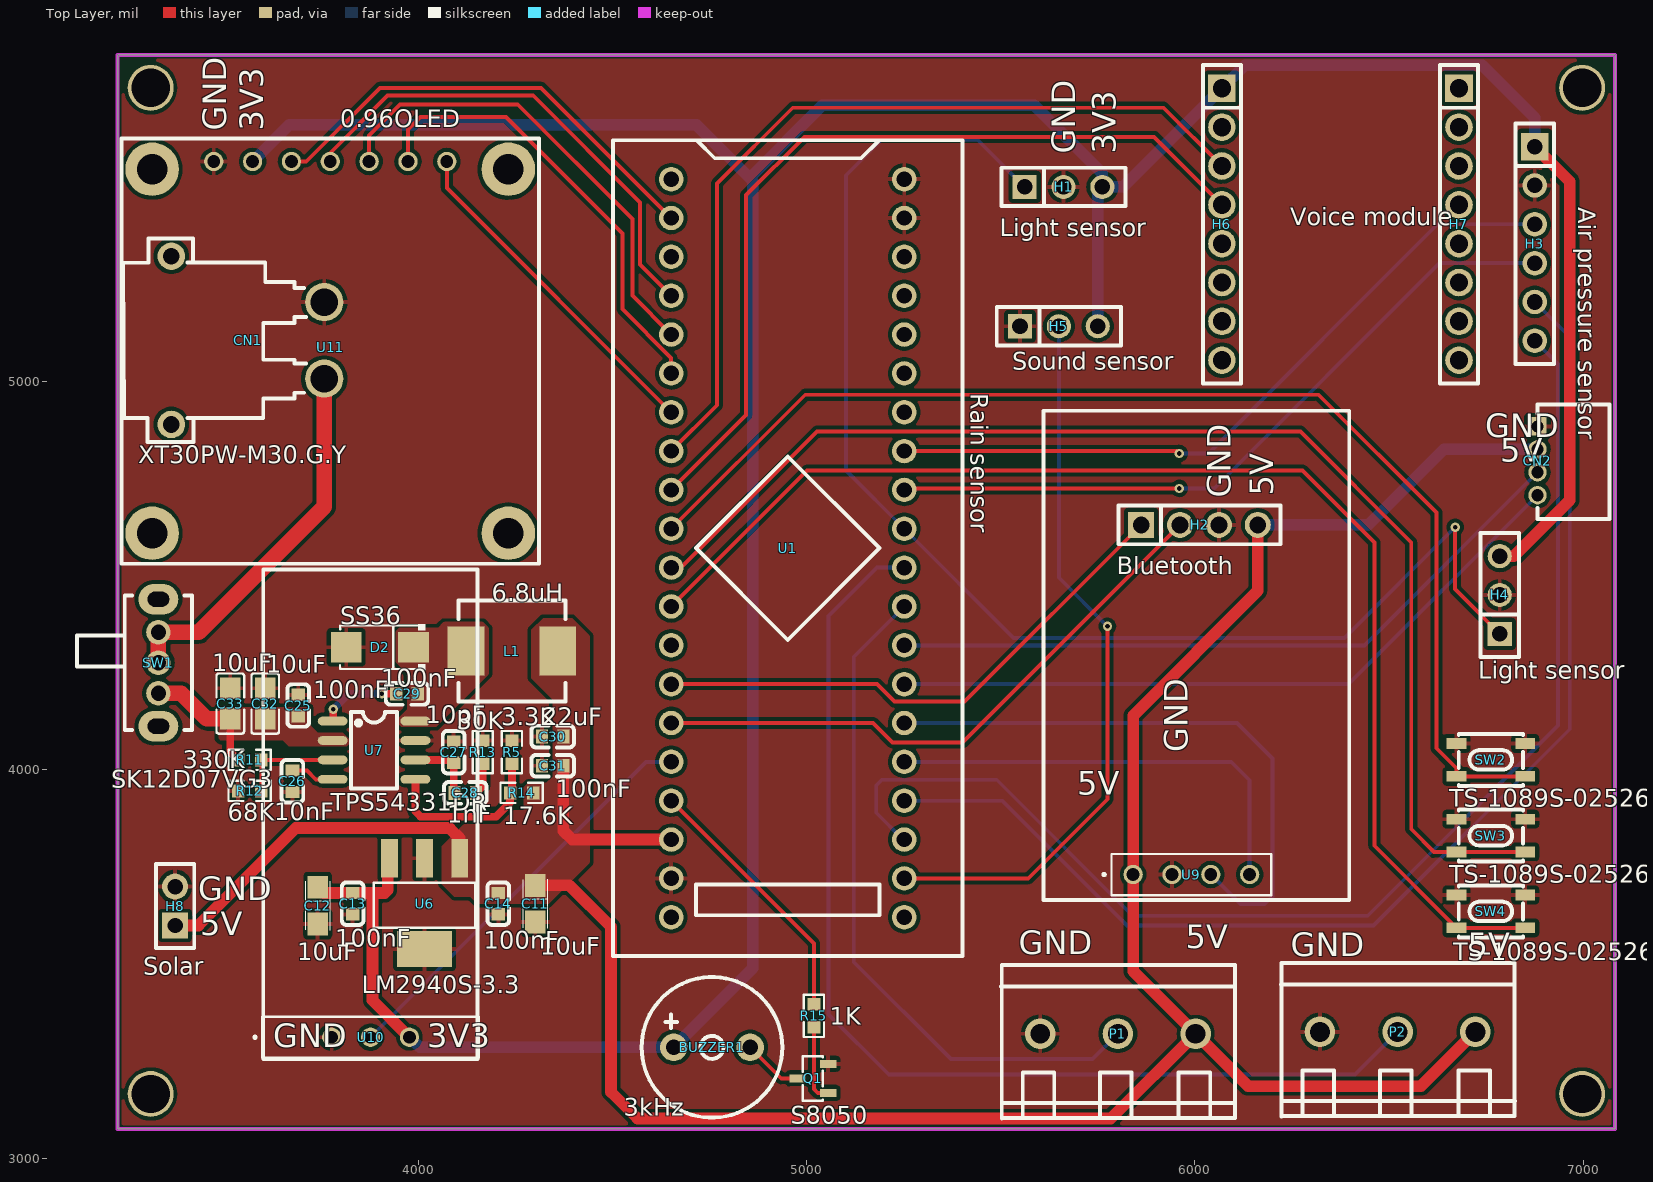
[diagram p0: Top Layer view]
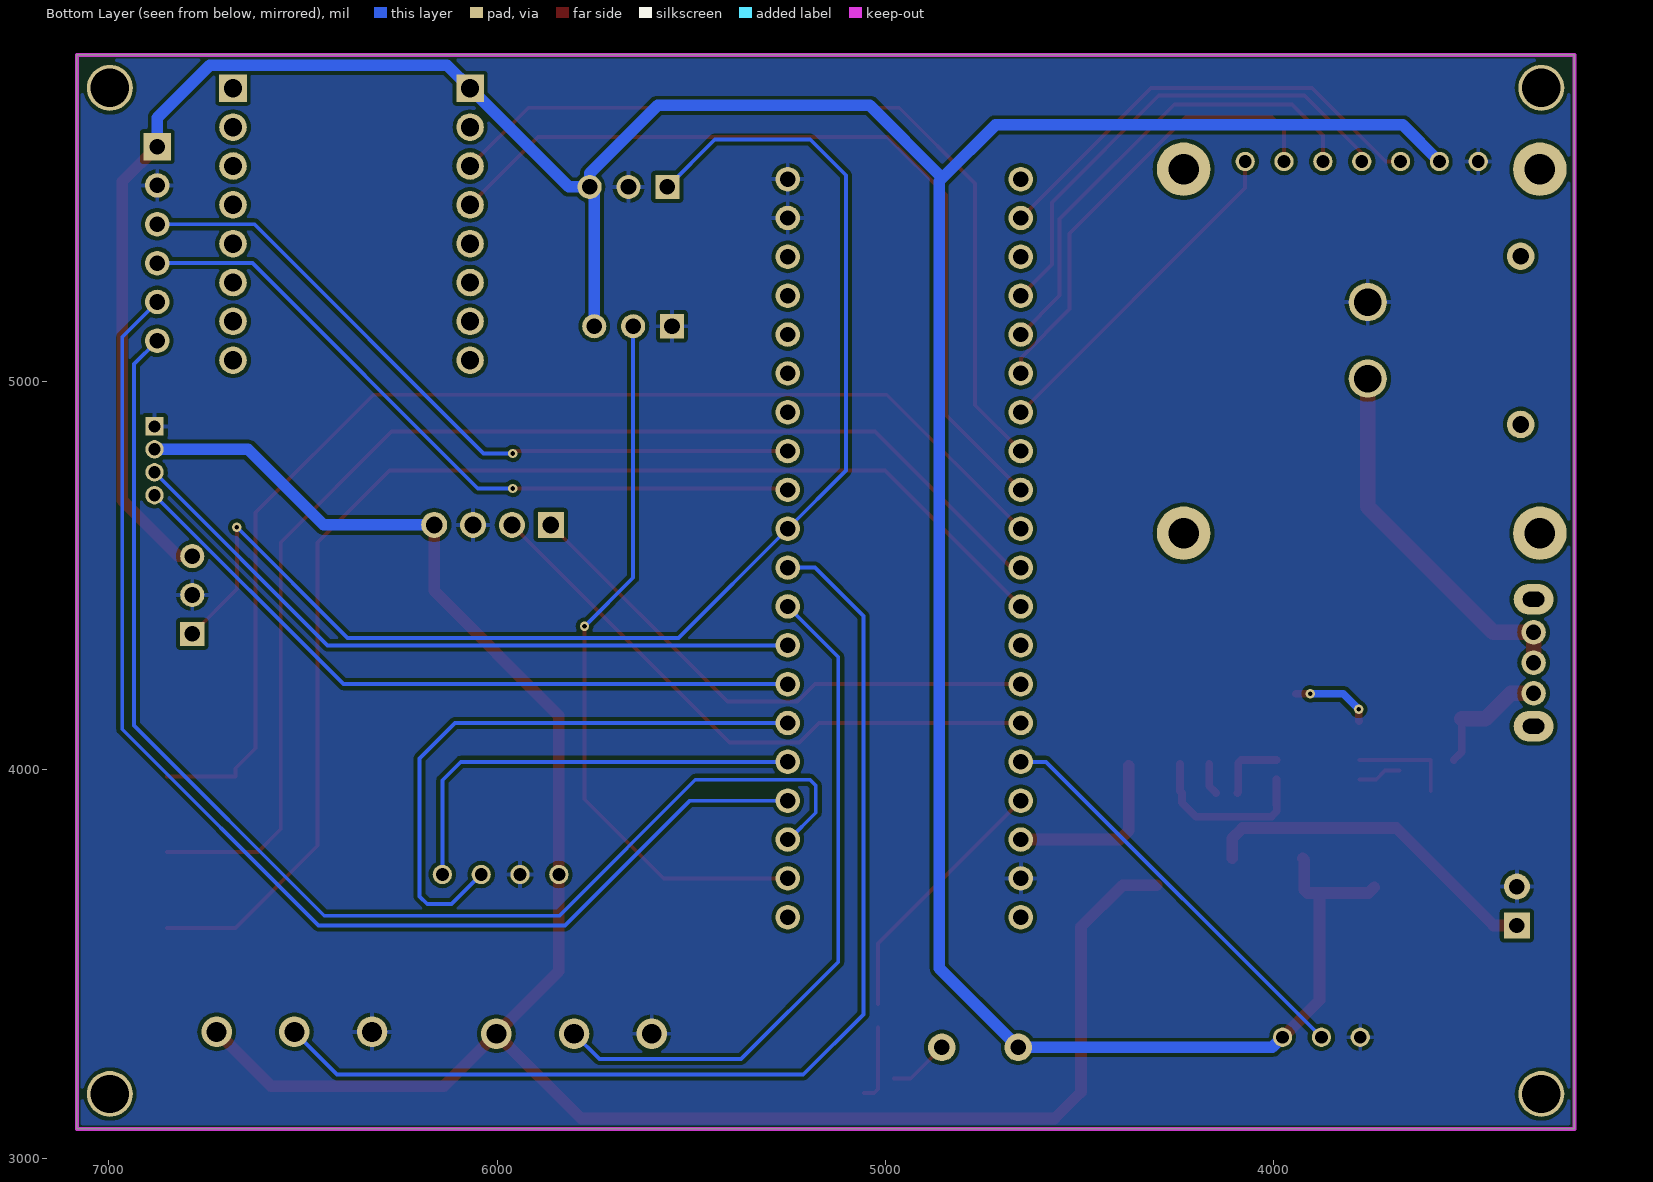
[diagram p1: Bottom Layer view, seen from below]
# Altium PCB MISC64781.pcbdoc
Units mil, origin at the board's own origin, x right, y up, seen from the top; angles counter-clockwise.
Board outline 3855 x 2765 mil, 2 copper layers (Top Layer, Bottom Layer), stack 62.206 mil thick; 45 components, 45 nets, 189 pads, 6 vias.

## Layer stack, top to bottom
Top Solder Mask Layer: solder mask 0.394, Dk 3.3
Top Layer: signal copper 1.379
Dielectric1: surface 59.449, FR4, Dk 4.5
Bottom Layer: signal copper 1.378
Bottom Solder Mask Layer: solder mask 0.394, Dk 3.3

## Board outline
3226.76,5840 3226.76,3075 7081.76,3075 7081.76,5840

## Design rules (kind name [scope] priority, off if disabled: settings)
BoardOutlineClearance copperThickness2oz_1 [All] p2 off: genericclearance=7.99 ignorepadtopadclearanceinfootprint=FALSE except(0: Arc-SplitContinuation Track-SplitContinuation SMDPad-SplitContinuation THPad-SplitContinuation Via-SplitContinuation Fill-SplitContinuation Region-SplitContinuation Poly-SplitContinuation Text-SplitContinuation Hole-SplitContinuation; 5.98: Arc-CutoutEdge Track-CutoutEdge SMDPad-CutoutEdge THPad-CutoutEdge Via-CutoutEdge Text-CutoutEdge; 6.89: Hole-OutlineEdge Hole-CutoutEdge; 10: Poly-OutlineEdge Poly-CutoutEdge; 11.81: Arc-OutlineEdge Track-OutlineEdge SMDPad-OutlineEdge THPad-OutlineEdge Via-OutlineEdge Fill-OutlineEdge Region-OutlineEdge Text-OutlineEdge Fill-CutoutEdge Region-CutoutEdge)
BoardOutlineClearance Plane_innerPlane_1 [All] p4 off: genericclearance=4.02 ignorepadtopadclearanceinfootprint=FALSE except(0: Arc-SplitContinuation Track-SplitContinuation SMDPad-SplitContinuation THPad-SplitContinuation Via-SplitContinuation Fill-SplitContinuation Region-SplitContinuation Poly-SplitContinuation Text-SplitContinuation Hole-SplitContinuation; 5.98: Arc-CutoutEdge Track-CutoutEdge SMDPad-CutoutEdge THPad-CutoutEdge Via-CutoutEdge Text-CutoutEdge; 6.89: Hole-OutlineEdge Hole-CutoutEdge; 10: Poly-OutlineEdge Poly-CutoutEdge; 11.81: Arc-OutlineEdge Track-OutlineEdge SMDPad-OutlineEdge THPad-OutlineEdge Via-OutlineEdge Fill-OutlineEdge Region-OutlineEdge Text-OutlineEdge Fill-CutoutEdge Region-CutoutEdge)
BoardOutlineClearance Copper_copperRegion_1 [All] p6 off: genericclearance=4.02 ignorepadtopadclearanceinfootprint=FALSE except(0: Arc-SplitContinuation Track-SplitContinuation SMDPad-SplitContinuation THPad-SplitContinuation Via-SplitContinuation Fill-SplitContinuation Region-SplitContinuation Poly-SplitContinuation Text-SplitContinuation Hole-SplitContinuation; 5.98: Arc-CutoutEdge Track-CutoutEdge SMDPad-CutoutEdge THPad-CutoutEdge Via-CutoutEdge Text-CutoutEdge; 6.89: Hole-OutlineEdge Hole-CutoutEdge; 10: Poly-OutlineEdge Poly-CutoutEdge; 11.81: Arc-OutlineEdge Track-OutlineEdge SMDPad-OutlineEdge THPad-OutlineEdge Via-OutlineEdge Fill-OutlineEdge Region-OutlineEdge Text-OutlineEdge Fill-CutoutEdge Region-CutoutEdge)
BoardOutlineClearance Copper_电源_1 [All] p8 off: genericclearance=4.02 ignorepadtopadclearanceinfootprint=FALSE except(0: Arc-SplitContinuation Track-SplitContinuation SMDPad-SplitContinuation THPad-SplitContinuation Via-SplitContinuation Fill-SplitContinuation Region-SplitContinuation Poly-SplitContinuation Text-SplitContinuation Hole-SplitContinuation; 5.98: Arc-CutoutEdge Track-CutoutEdge SMDPad-CutoutEdge THPad-CutoutEdge Via-CutoutEdge Text-CutoutEdge; 6.89: Hole-OutlineEdge Hole-CutoutEdge; 10: Poly-OutlineEdge Poly-CutoutEdge; 11.81: Arc-OutlineEdge Track-OutlineEdge SMDPad-OutlineEdge THPad-OutlineEdge Via-OutlineEdge Fill-OutlineEdge Region-OutlineEdge Text-OutlineEdge Fill-CutoutEdge Region-CutoutEdge)
BoardOutlineClearance copperThickness1oz_1 [All] p10: genericclearance=4.02 ignorepadtopadclearanceinfootprint=FALSE except(0: Arc-SplitContinuation Track-SplitContinuation SMDPad-SplitContinuation THPad-SplitContinuation Via-SplitContinuation Fill-SplitContinuation Region-SplitContinuation Poly-SplitContinuation Text-SplitContinuation Hole-SplitContinuation; 5.98: Arc-CutoutEdge Track-CutoutEdge SMDPad-CutoutEdge THPad-CutoutEdge Via-CutoutEdge Text-CutoutEdge; 6.89: Hole-OutlineEdge Hole-CutoutEdge; 10: Poly-OutlineEdge Poly-CutoutEdge; 11.81: Arc-OutlineEdge Track-OutlineEdge SMDPad-OutlineEdge THPad-OutlineEdge Via-OutlineEdge Fill-OutlineEdge Region-OutlineEdge Text-OutlineEdge Fill-CutoutEdge Region-CutoutEdge)
Clearance copperThickness2oz [All] p1 off: gap=7.99 ignorepadtopadclearanceinfootprint=FALSE except(5.98: SMDPad-Track SMDPad-SMDPad THPad-Track SMDPad-THPad THPad-THPad Track-Via SMDPad-Via THPad-Via Via-Via Fill-SMDPad Region-SMDPad Fill-THPad Region-THPad Fill-Via Region-Via Fill-Fill Fill-Region Region-Region Arc-Track Arc-SMDPad Arc-THPad Arc-Via Fill-Arc Region-Arc Arc-Arc Text-Track SMDPad-Text Text-THPad Text-Via Fill-Text Region-Text Arc-Text Text-Text; 6.89: Hole-Track Hole-SMDPad Hole-THPad Hole-Via Fill-Hole Region-Hole Hole-Arc Hole-Text; 10: Poly-Track Poly-SMDPad Poly-THPad Poly-Via Poly-Fill Poly-Region Poly-Poly Poly-Arc Poly-Text Poly-Hole; 11.81: Fill-Track Region-Track)
Clearance Plane_innerPlane [All] p3 off: gap=4.02 ignorepadtopadclearanceinfootprint=FALSE except(5.98: SMDPad-Track SMDPad-SMDPad THPad-Track SMDPad-THPad THPad-THPad Track-Via SMDPad-Via THPad-Via Via-Via Fill-SMDPad Region-SMDPad Fill-THPad Region-THPad Fill-Via Region-Via Fill-Fill Fill-Region Region-Region Arc-Track Arc-SMDPad Arc-THPad Arc-Via Fill-Arc Region-Arc Arc-Arc Text-Track SMDPad-Text Text-THPad Text-Via Fill-Text Region-Text Arc-Text Text-Text; 6.89: Hole-Track Hole-SMDPad Hole-THPad Hole-Via Fill-Hole Region-Hole Hole-Arc Hole-Text; 10: Poly-Track Poly-SMDPad Poly-THPad Poly-Via Poly-Fill Poly-Region Poly-Poly Poly-Arc Poly-Text Poly-Hole; 11.81: Fill-Track Region-Track)
Clearance Copper_copperRegion [All] p5 off: gap=4.02 ignorepadtopadclearanceinfootprint=FALSE except(5.98: SMDPad-Track SMDPad-SMDPad THPad-Track SMDPad-THPad THPad-THPad Track-Via SMDPad-Via THPad-Via Via-Via Fill-SMDPad Region-SMDPad Fill-THPad Region-THPad Fill-Via Region-Via Fill-Fill Fill-Region Region-Region Arc-Track Arc-SMDPad Arc-THPad Arc-Via Fill-Arc Region-Arc Arc-Arc Text-Track SMDPad-Text Text-THPad Text-Via Fill-Text Region-Text Arc-Text Text-Text; 6.89: Hole-Track Hole-SMDPad Hole-THPad Hole-Via Fill-Hole Region-Hole Hole-Arc Hole-Text; 10: Poly-Track Poly-SMDPad Poly-THPad Poly-Via Poly-Fill Poly-Region Poly-Poly Poly-Arc Poly-Text Poly-Hole; 11.81: Fill-Track Region-Track)
Clearance Copper_电源 [All] p7 off: gap=4.02 ignorepadtopadclearanceinfootprint=FALSE except(5.98: SMDPad-Track SMDPad-SMDPad THPad-Track SMDPad-THPad THPad-THPad Track-Via SMDPad-Via THPad-Via Via-Via Fill-SMDPad Region-SMDPad Fill-THPad Region-THPad Fill-Via Region-Via Fill-Fill Fill-Region Region-Region Arc-Track Arc-SMDPad Arc-THPad Arc-Via Fill-Arc Region-Arc Arc-Arc Text-Track SMDPad-Text Text-THPad Text-Via Fill-Text Region-Text Arc-Text Text-Text; 6.89: Hole-Track Hole-SMDPad Hole-THPad Hole-Via Fill-Hole Region-Hole Hole-Arc Hole-Text; 10: Poly-Track Poly-SMDPad Poly-THPad Poly-Via Poly-Fill Poly-Region Poly-Poly Poly-Arc Poly-Text Poly-Hole; 11.81: Fill-Track Region-Track)
Clearance copperThickness1oz [All] p9: gap=4.02 ignorepadtopadclearanceinfootprint=FALSE except(5.98: SMDPad-Track SMDPad-SMDPad THPad-Track SMDPad-THPad THPad-THPad Track-Via SMDPad-Via THPad-Via Via-Via Fill-SMDPad Region-SMDPad Fill-THPad Region-THPad Fill-Via Region-Via Fill-Fill Fill-Region Region-Region Arc-Track Arc-SMDPad Arc-THPad Arc-Via Fill-Arc Region-Arc Arc-Arc Text-Track SMDPad-Text Text-THPad Text-Via Fill-Text Region-Text Arc-Text Text-Text; 6.89: Hole-Track Hole-SMDPad Hole-THPad Hole-Via Fill-Hole Region-Hole Hole-Arc Hole-Text; 10: Poly-Track Poly-SMDPad Poly-THPad Poly-Via Poly-Fill Poly-Region Poly-Poly Poly-Arc Poly-Text Poly-Hole; 11.81: Fill-Track Region-Track)
DiffPairsRouting differentialPair [All] p1: maxlimit=6 minlimit=6 mostfreqgap=6 toplayer_minwidth=5 toplayer_prefwidth=10 toplayer_maxwidth=100 toplayer_mingap=6 toplayer_prefgap=6 toplayer_maxgap=6 bottomlayer_minwidth=5 bottomlayer_prefwidth=10 bottomlayer_maxwidth=100 bottomlayer_mingap=6 bottomlayer_prefgap=6 bottomlayer_maxgap=6 maxuncoupledlength=10
HoleToHoleClearance otherClearance [All] p1: gap=11.81 allowstackedmicrovias=TRUE
Length netLength [All] p1: minlimit=0 maxlimit=0
PasteMaskExpansion pasteMaskExpansion [All] p1: expansion=0
PlaneConnect innerPlane [All] p1: planeconnectstyle=Relief reliefexpansion=20 reliefentries=4 reliefconductorwidth=10 reliefairgap=10
PolygonConnect 电源 [All] p1 off: connectstyle=Direct reliefconductorwidth=10 reliefentries=4 polygonreliefangle="90 Angle" airgapwidth=10 via.connectstyle=Relief via.reliefconductorwidth=10 via.reliefentries=4 via.polygonreliefangle="90 Angle" via.airgapwidth=10
PolygonConnect copperRegion [All] p2: connectstyle=Relief reliefconductorwidth=10 reliefentries=4 polygonreliefangle="90 Angle" airgapwidth=10 via.connectstyle=Relief via.reliefconductorwidth=10 via.reliefentries=4 via.polygonreliefangle="90 Angle" via.airgapwidth=10
RoutingVias viaSize [All] p1: holewidth=12.01 width=24.02 viastyle="Through Hole" minholewidth=11.81 minwidth=19.68 maxholewidth=248.03 maxwidth=393.7
SolderMaskExpansion solderMaskExpansion [IsVia] p1: expansion=-1000 istentingtop=TRUE
SolderMaskExpansion solderMaskExpansion [All] p2: expansion=2.01 istentingtop=FALSE
Width copperThickness2oz_2 [All] p1 off: maxlimit=100 minlimit=8 preferedwidth=10
Width copperThickness1oz_2 [All] p2: maxlimit=100 minlimit=5 preferedwidth=10

## Components (designator, comment, footprint, x,y, rotation, side; value= is the part's Value field where it differs from the comment)
BUZZER1 "3kHz" BUZ-TH_BD9.0-P5.00-D0.6-FD 4756.76,3285 r0 top
C11 "10uF" CASE-A_3216 4301.76,3655 r270 top
C12 "10uF" CASE-A_3216 3741.76,3650 r270 top
C13 "100nF" C0603 3831.76,3655 r90 top
C14 "100nF" C0603 4206.76,3655 r270 top
C25 "100nF" C0603 3691.76,4165 r270 top
C26 "10nF" C0603 3676.76,3970 r90 top
C27 "10pF" C0603 4091.76,4045 r270 top
C28 "1nF" C0603 4121.76,3940 r180 top
C29 "100nF" C0603 3971.76,4195 r0 top
C30 "22uF" C0603 4346.76,4085 r0 top
C31 "100nF" C0603 4346.76,4010 r0 top
C32 "10uF" C0805 3606.76,4170 r270 top
C33 "10uF" C0805 3516.76,4170 r270 top
CN1 "XT30PW-M30.G.Y" CONN-TH_XT30PW-M 3561.76,5105 r270 top
CN2 "PM2.5 sensor" CONN-TH_4P-P1.50_HCTL_HC-ZH1.5-4AW 6881.76,4795 r90 top
D2 "SS36" SMA_L4.3-W2.6-LS5.2-RD 3901.76,4315 r180 top
H1 "Light sensor" HDR-TH_3P-P2.54-V-F 5661.76,5500 r0 top
H2 "Bluetooth" HDR-TH_4P-P2.54-V-F 6011.76,4630 r0 top
H3 "Air pressure sensor" HDR-TH_6P-P2.54-V-F 6874.74,5353.84 r270 top
H4 "Light sensor" HDR-TH_3P-P2.54-V-F 6784.74,4449.51 r90 top
H5 "Sound sensor" HDR-TH_3P-P2.54-V-F 5649.74,5141.4 r0 top
H6 "Voice module" HDR-TH_8P-P2.54-V-F-1 6069.49,5403.84 r270 top
H7 "" HDR-TH_8P-P2.54-V-F-1 6679.74,5403.84 r270 top
H8 "Solar" HDR-TH_2P-P2.54-V-F 3374.74,3648.84 r90 top
L1 "6.8uH" IND-SMD_L7.0-W6.6 4241.76,4305 r0 top
P1 "Wind speed sensor" CONN-TH_3P-P5.00_WJ500V-5.08-3P 5801.76,3320 r0 top
P2 "Wind direction sensor" CONN-TH_3P-P5.00_WJ500V-5.08-3P 6521.76,3325 r0 top
Q1 "S8050" SOT-23-3_L2.9-W1.3-P1.90-LS2.3-BR 5016.76,3205 r0 top
R5 "3.3K" R0603 4241.76,4045 r270 top
R11 "330K" R0603 3566.76,4025 r180 top
R12 "68K" R0603 3566.76,3945 r0 top
R13 "30K" R0603 4166.76,4045 r270 top
R14 "17.6K" R0603 4266.76,3940 r0 top
R15 "1K" R0603 5019.16,3366.32 r270 top
SW1 "SK12D07VG3" SW-TH_SK12D07VG3 3331.76,4275 r270 top
SW2 "TS-1089S-02526" SW-SMD_4P-L4.2-W3.3-P2.15-LS5.1 6761.76,4025 r0 top
SW3 "TS-1089S-02526" SW-SMD_4P-L4.2-W3.3-P2.15-LS5.1 6761.76,3830 r0 top
SW4 "TS-1089S-02526" SW-SMD_4P-L4.2-W3.3-P2.15-LS5.1 6761.76,3635 r0 top
U1 "LCKFB-DKX-STM32F103C8T6" CONN-TH_L53.3-W22.9_STM32F103C8T6-CARD 4951.76,4570 r270 top
U6 "LM2940S-3.3" SOT-223-3_L6.5-W3.4-P2.30-LS7.0-BR 4016.76,3655 r90 top
U7 "TPS54331DR" SOIC-8_L5.0-W4.0-P1.27-LS6.0-BL 3886.76,4050 r270 top
U9 "Rain sensor" MQ-2烟雾传感器模块 5609.74,4923.84 r270 top
U10 "DHT11 temperature and humidity sensor" DHT11温湿度模块 3601.76,4515 r270 top
U11 "0.96OLED" 0.96寸OLED 3236.76,4530 r0 top

## Footprints (in the part's own frame and the unit in brackets; to place one, negate y for a bottom-side part, rotate by r counter-clockwise, add the part's x,y. Pads: shape width x height; smd on the part's side, far side on the other; paste and mask are expansions set on the pad)
0.96寸OLED [mm]
  round 1.26 hole 0.84: 1(6.03,26.3) 2(8.57,26.3) 3(11.11,26.3) 4(13.65,26.3) 5(16.19,26.3) 6(18.73,26.3) 7(21.27,26.3)
  round 3.5 hole 2: 8(2,25.8) 9(25.3,25.8) 10(2,2) 11(25.3,2)
  silkscreen extent 0,0 27.3,27.8
BUZ-TH_BD9.0-P5.00-D0.6-FD [mm]
  round 1.8 hole 1 copper offset 0,0: 1(-2.5,0)
  round 1.8 hole 1: 2(2.5,0)
  silkscreen extent -4.6,-4.6 4.6,4.6
C0603 [mm]
  rect 0.8x0.9 smd: 1(-0.7,0) 2(0.7,0)
  silkscreen extent -1.39,-0.71 1.39,0.71
C0805 [mm]
  rect 1.41x1.35 smd paste-100 mask+0.051: 1(-1,0) 2(1,0)
  silkscreen extent -1.96,-0.9 1.96,0.9
CASE-A_3216 [mil]
  rect 59.05x53.5 smd: 1(-47.24,0) 2(47.24,0)
  silkscreen extent -63,-32 63,32
CONN-TH_3P-P5.00_WJ500V-5.08-3P [mm]
  round 2 hole 1.3: 1(-5.08,0) 2(0,0) 3(5.08,0)
  silkscreen extent -7.64,-5.53 7.66,4.5
CONN-TH_4P-P1.50_HCTL_HC-ZH1.5-4AW [mm]
  round 1.2 hole 0.8 paste+0 mask+0.05: 1(-2.25,0) 2(-0.75,0) 3(0.75,0)
  rect 1.2x1.2 hole 0.8 paste+0 mask+0.05: 4(2.25,0)
  silkscreen extent -3.81,-4.7 3.68,0
CONN-TH_L53.3-W22.9_STM32F103C8T6-CARD [mm]
  round 1.6 hole 1: 1(-24.13,-7.62) 2(-21.59,-7.62) 3(-19.05,-7.62) 4(-16.51,-7.62) 5(-13.97,-7.62) 6(-11.43,-7.62) 7(-8.89,-7.62) 8(-6.35,-7.62) 9(-3.81,-7.62) 10(-1.27,-7.62) 11(1.27,-7.62) 12(3.81,-7.62) 13(6.35,-7.62) 14(8.89,-7.62) 15(11.43,-7.62) 16(13.97,-7.62) 17(16.51,-7.62) 18(19.05,-7.62) 19(21.59,-7.62) 20(24.13,-7.62) 21(24.13,7.62) 22(21.59,7.62) 23(19.05,7.62) 24(16.51,7.62) 25(13.97,7.62) 26(11.43,7.62) 27(8.89,7.62) 28(6.35,7.62) 29(3.81,7.62) 30(1.27,7.62) 31(-1.27,7.62) 32(-3.81,7.62) 33(-6.35,7.62) 34(-8.89,7.62) 35(-11.43,7.62) 36(-13.97,7.62) 37(-16.51,7.62) 38(-19.05,7.62) 39(-21.59,7.62) 40(-24.13,7.62)
  silkscreen extent -26.67,-11.43 26.67,11.43
CONN-TH_XT30PW-M [mm]
  round 2.5 hole 1.8: 1(-2.5,5) 2(2.5,5)
  round 1.8 hole 1.1: 3(5.5,-5) 4(-5.5,-5)
  silkscreen extent -6.65,-8.15 6.65,3.81
DHT11温湿度模块 [mil]
  round 49.61 hole 33.07: 1(1203.85,376.15) 2(1203.85,276.15) 3(1203.85,176.15)
  silkscreen extent 0,-28 1260,555
HDR-TH_2P-P2.54-V-F [mm]
  rect 1.7x1.7 hole 1: 1(-1.27,0)
  round 1.7 hole 1: 2(1.27,0)
  silkscreen extent -2.74,-1.25 2.74,1.25
HDR-TH_3P-P2.54-V-F [mil]
  rect 62x62 hole 40.16: 1(-100,0)
  round 62 hole 40.16: 2(0,0) 3(100,0)
  silkscreen extent -160,-49 160,49
HDR-TH_4P-P2.54-V-F [mm]
  rect 1.7x1.7 hole 1.1: 1(-3.81,0)
  round 1.7 hole 1.1: 2(-1.27,0) 3(1.27,0) 4(3.81,0)
  silkscreen extent -5.29,-1.27 5.29,1.27
HDR-TH_6P-P2.54-V-F [mm]
  rect 1.8x1.8 hole 1.02: 1(-6.35,0)
  round 1.6 hole 1.02: 2(-3.81,0) 3(-1.27,0) 4(1.27,0) 5(3.81,0) 6(6.35,0)
  silkscreen extent -7.87,-1.25 7.87,1.25
HDR-TH_8P-P2.54-V-F-1 [mm]
  rect 1.8x1.8 hole 1.2: 1(-8.89,0)
  round 1.8 hole 1.2: 2(-6.35,0) 3(-3.81,0) 4(-1.27,0) 5(1.27,0) 6(3.81,0) 7(6.35,0) 8(8.89,0)
  silkscreen extent -10.41,-1.25 10.41,1.25
IND-SMD_L7.0-W6.6 [mm]
  rect 2.4x3.2 smd: 1(-3,0) 2(3,0)
  silkscreen extent -3.5,-3.3 3.5,3.3
MQ-2烟雾传感器模块 [mil]
  round 49.61 hole 33.07: 1(1193.85,231.15) 2(1193.85,331.15) 3(1193.85,431.15) 4(1193.85,531.15)
  silkscreen extent 0,0 1260,787
R0603 [mil]
  rect 31.75x34.02 smd paste-3937.01 mask+2: 1(-29.66,0) 2(29.66,0)
  silkscreen extent -55,-26 55,26
SMA_L4.3-W2.6-LS5.2-RD [mm]
  rect 2x2 smd: 1(-2.2,0) 2(2.2,0)
  silkscreen extent -2.98,-1.5 2.6,1.5
SOIC-8_L5.0-W4.0-P1.27-LS6.0-BL [mil]
  oval 22.38x76.78 smd: 1(-75,-106.5) 2(-25,-106.5) 3(25,-106.5) 4(75,-106.5) 5(75,106.5) 6(25,106.5) 7(-25,106.5) 8(-75,106.5)
  silkscreen extent -98,-59 98,59
SOT-23-3_L2.9-W1.3-P1.90-LS2.3-BR [mm]
  rect 1.07x0.532 smd: 1(0.99,-0.95) 2(0.99,0.95) 3(-0.99,0)
  silkscreen extent -0.66,-1.45 0.64,1.45
SOT-223-3_L6.5-W3.4-P2.30-LS7.0-BR [mm]
  rect 2.5x1.1 smd: 1(2.97,-2.3) 2(2.97,0) 3(2.97,2.3)
  rect 2.34x3.6 smd: 4(-2.97,0)
  silkscreen extent -1.57,-3.33 1.37,3.33
SW-SMD_4P-L4.2-W3.3-P2.15-LS5.1 [mm]
  rect 1.3x0.7 smd: 1(-2.25,1.075) 2(2.25,1.075) 3(-2.25,-1.075) 4(2.25,-1.075)
  silkscreen extent -2.1,-1.7 2.1,1.7
SW-TH_SK12D07VG3 [mm]
  round 1.6 hole 1: 1(-2,0) 2(0,0) 3(2,0)
  oval 2x2.6 hole 1 slot 1.4 at 90 deg: 4(4.15,0) 5(-4.15,0)
  silkscreen extent -4.4,-5.33 4.4,2.2

## Free pads (board coordinates)
  round 118.11 hole 98.43: 1(3311.76,3165) 1(3311.76,5755) 1(6996.76,3165) 1(6996.76,5755)

## Via types
v1: diameter 24.02, hole 12, Top Layer to Bottom Layer, 6 vias

## Nets (pads, with @x,y where several pads share a name; then routed paths per layer and width w, separated by ;. In a path a pad name is that pad's centre, name@x,y a point inside that pad or via, vN(x,y) a via of type N, cw(c..) or ccw(c..) an arc to the next point about the centre after c; other vN are vias at no path point)
3V3: BUZZER1.1 C12.1 C13.2 H1.3 H3.1 H4.3 H5.3 H6.1 U6.3 U10.1 U11.2 | length 9092.7
  Top Layer w30: C12.1 3756.44,3682.56 C13.2 3882.95,3682.56 ; U6.3 3921.76,3767.48 3921.76,3690 3914.32,3682.56 3882.95,3682.56 ; U10.1 3882.95,3406.11 3882.95,3682.56 ; H4.3 6820.41,4549.51 6964.74,4693.84 6964.74,5513.84 H3.1
  Bottom Layer w30: U11.2 3668.73,5660 4716.76,5660 4853.65,5523.11 ; U10.1 4004.06,3285 BUZZER1.1 4861.76,3488.43 4861.76,5515 4853.65,5523.11 ; H5.3 5749.74,5487.98 H1.3 ; H3.1 6874.74,5678.19 6739.74,5813.19 6128.85,5813.19 H6.1 5815.66,5500 H1.3 ; 4853.65,5523.11 5040.54,5710 5586.76,5710 5761.76,5535 H1.3
$1N560: BUZZER1.2 Q1.3 | length 155.7
  Top Layer w10: BUZZER1.2 4935.19,3205 Q1.3
$1N563: Q1.1 R15.2 | length 199.8
  Top Layer w10: R15.2 5019.16,3177.6 5029.16,3167.6 Q1.1
$1N2014: C26.2 U7.4 | length 112.8
  Top Layer w10: C26.2 3714.2,3997.56 3736.76,3975 U7.4
$1N2015: C27.2 C28.2 U7.6 | length 180.1
  Top Layer w20: U7.6 4084.2,4025 C27.2 4091.76,3942.44 C28.2
$1N2016: C28.1 R13.2 | length 82.6
  Top Layer w20: C28.1 4166.76,3957.44 R13.2
$1N2017: C29.2 D2.1 L1.1 U7.8
$1N2018: C29.1 U7.1 | length 209.6
  Top Layer w20: U7.1 3781.76,4126.5 v1(3781.76,4155) ; v1(3906.76,4195) C29.1
  Bottom Layer w20: v1(3781.76,4155) 3821.76,4195 v1(3906.76,4195)
$1N2020: R5.2 R14.1 U7.5 | length 449.7
  Top Layer w20: U7.5 3993.26,3909.78 3992.62,3909.14 3992.62,3892.98 4006.76,3878.84 4200.6,3878.84 4237.1,3915.34 R14.1 4241.76,3944.66 R5.2
$1N2028: R11.1 R12.2 U7.3 | length 263.8
  Top Layer w10: R12.2 R11.1 U7.3
+5V: C11.1 C14.1 C30.2 C31.2 CN2.3 H2.4 H8.1 L1.2 P1.3 P2.3 R14.2 U1.18 U6.1 U9.1 | length 6785.3
  Top Layer w30: H8.1 3434.74,3598.84 3685.73,3849.82 4080.9,3849.82 4107.31,3823.41 U6.1 ; C11.1 4389.52,3702.24 4496.76,3595 4496.76,3170 4564.95,3101.81 5783.57,3101.81 P1.3 ; C31.2 4374.32,3842.44 4396.76,3820 U1.18 ; H2.4 6161.76,4460 5840.89,4139.13 U9.1 5840.89,3480.87 P1.3 ; P2.3 6581.76,3185 6136.76,3185 P1.3
  Bottom Layer w30: H2.4 6446.76,4630 6641.29,4824.53 CN2.3
BEEP: R15.1 U1.17 | length 676.2
  Top Layer w10: U1.17 5019.16,3552.6 R15.1
CSB: H3.5 U1.24 | length 3192.5
  Bottom Layer w10: U1.24 5503.58,3920 5824.74,3598.84 6459.74,3598.84 6964.74,4103.84 6964.74,5113.84 H3.5
DHT_DATA: U1.16 U10.2 | length 1067.5
  Bottom Layer w10: U10.2 4586.76,4020 U1.16
FS_ADC: P1.2 U1.29 | length 1779.3
  Bottom Layer w10: U1.29 5121.76,4290 5121.76,3505 5371.76,3255 5736.76,3255 P1.2
FX_ADC: P2.2 U1.30 | length 2846.5
  Bottom Layer w10: U1.30 5181.76,4520 5056.76,4395 5056.76,3370 5211.76,3215 6411.76,3215 P2.2
GND: H6.5
GZ_ADC: H1.1 H4.1 U1.31 | length 3495.3
  Top Layer w10: v1(6669.74,4623.84) 6669.74,4464.51 H4.1
  Bottom Layer w10: H1.1 5439.69,5622.07 5193.83,5622.07 5101.76,5530 5101.76,4770 U1.31 5532.92,4338.84 6384.74,4338.84 v1(6669.74,4623.84)
KEY1: SW2.3 SW2.4 U1.10 | length 3115.8
  Top Layer w10: U1.10 4996.76,4965 6318.16,4965 6621.76,4661.4 6621.76,4055 6673.18,4003.58 SW2.3 SW2.4
KEY2: SW3.3 SW3.4 U1.11 | length 3224.3
  Top Layer w10: U1.11 4676.76,4520 5026.76,4870 6271.76,4870 6556.76,4585 6556.76,3846.82 6615.9,3787.68 SW3.3 SW3.4
KEY3: SW4.3 SW4.4 U1.12 | length 3288.7
  Top Layer w10: U1.12 5001.76,4770 6276.76,4770 6461.76,4585 6461.76,3804.09 SW4.3 SW4.4
MQ_A0: U1.25 U9.4 | length 1151.4
  Bottom Layer w10: U1.25 6093.58,4020 6140.89,3972.69 U9.4
MQ_D0: U1.26 U9.3 | length 1539.4
  Bottom Layer w10: U1.26 6108.58,4120 6199.74,4028.84 6199.74,3673.84 6179.74,3653.84 6117.04,3653.84 U9.3
OLED_CS: U1.7 U11.7 | length 884.7
  Top Layer w10: U11.7 4074.16,5497.6 U1.7
OLED_DC: U1.6 U11.6 | length 1184.1
  Top Layer w10: U11.6 3974.16,5647.4 4006.76,5680 4226.76,5680 4526.28,5380.48 4526.28,5185.4 4651.76,5059.92 U1.6
OLED_RES: U1.5 U11.5 | length 1238.3
  Top Layer w10: U11.5 3874.16,5632.4 3953.83,5712.07 4256.76,5712.07 4551.76,5417.07 4551.76,5220 U1.5
PC13: H5.2 U1.22 | length 1876.8
  Top Layer w10: U1.22 5570.9,3720 5774.74,3923.84 v1(5774.74,4368.84)
  Bottom Layer w10: H5.2 5649.74,4493.84 v1(5774.74,4368.84)
PGND: C11.2 C12.2 C13.1 C14.2 C25.1 C26.1 C27.1 C30.1 C31.1 C32.1 C33.1 CN1.1 CN2.4 D2.2 H1.2 H2.3 H3.2 H4.2 H5.1 H8.2 P1.1 P2.1 Q1.2 R5.1 R12.1 R13.1 SW2.1 SW2.2 SW3.1 SW3.2 SW4.1 SW4.2 U1.19 U1.39 U1.40 U6.2 U6.4 U7.7 U9.2 U10.3 U11.1
RX: H6.3 U1.8 | length 2180.4
  Top Layer w10: U1.8 4769.74,4937.98 4769.74,5508.84 4964.74,5703.84 5919.49,5703.84 H6.3
SCL: H3.3 U1.33 | length 1869.9
  Top Layer w10: U1.33 5953.58,4820 v1(5959.74,4813.84)
  Bottom Layer w10: v1(5959.74,4813.84) 6034.74,4813.84 6624.74,5403.84 H3.3
SDA: H3.4 U1.32 | length 1864.8
  Top Layer w10: U1.32 5255.6,4723.84 v1(5959.74,4723.84)
  Bottom Layer w10: v1(5959.74,4723.84) 6049.74,4723.84 6629.74,5303.84 H3.4
SDO: H3.6 U1.23 | length 3294.5
  Bottom Layer w10: U1.23 5248.58,3820 5179.74,3888.84 5179.74,3958.84 5194.74,3973.84 5489.74,3973.84 5839.74,3623.84 6444.74,3623.84 6934.74,4113.84 6934.74,5043.84 H3.6
SPI2_MISO: U1.3
SPI2_MOSI: U1.4 U11.4 | length 1267.8
  Top Layer w10: U11.4 3774.16,5587.4 3921.76,5735 4296.76,5735 4571.76,5460 4571.76,5300 U1.4
SPI2_NSS: U1.1
SPI2_SCK: U1.2 U11.3 | length 1194.9
  Top Layer w10: U11.3 3712.19,5565.43 3901.76,5755 4316.76,5755 U1.2
TX: H6.4 U1.9 | length 2198.1
  Top Layer w10: U1.9 4844.74,4912.98 4844.74,5478.84 4994.74,5628.84 5894.49,5628.84 H6.4
USART1_RX: H2.2 U1.15 | length 1562.7
  Top Layer w10: U1.15 5171.76,4120 5221.76,4070 5401.76,4070 H2.2
USART1_TX: H2.1 U1.14 | length 1417.1
  Top Layer w10: U1.14 5181.76,4220 5226.76,4175 5406.76,4175 H2.1
USART2_RX: CN2.2 U1.28 | length 1814.5
  Bottom Layer w10: U1.28 6436.29,4320 CN2.2
USART2_TX: CN2.1 U1.27 | length 1831.5
  Bottom Layer w10: U1.27 6395.35,4220 CN2.1
USART3_RX: U1.36
USART3_TX: U1.35
VBAT: CN1.2 SW1.1 SW1.2 | length 969.1
  Top Layer w40: SW1.2 SW1.1 3435.5,4353.74 3758.61,4676.85 CN1.2
VBAT_KEY: C25.2 C32.2 C33.2 R11.2 SW1.3 U7.2 | length 326.2
  Top Layer w20: C33.2 3516.76,4045.34 R11.2
  Top Layer w40: SW1.3 3390.5,4196.26 3456.13,4130.63 C33.2
pads on no net: CN1.3 CN1.4 H6.2 H6.6 H6.7 H6.8 H7.1 H7.2 H7.3 H7.4 H7.5 H7.6 H7.7 H7.8 SW1.4 SW1.5 U1.13 U1.20 U1.21 U1.34 U1.37 U1.38 U11.8 U11.9 U11.10 U11.11

## Polygon pours and split planes (outlines as drawn)
PGND on Top Layer (solid, remove dead copper, pour order 6): 3171.76,5895 3171.76,3010 7141.76,3010 7141.76,5895
VBAT_KEY on Top Layer (solid, remove dead copper, pour order 0): 3486.76,4160 3719.7,4160 3719.7,4117.06 3741.76,4095 3806.76,4095 3821.76,4080 3821.76,4065 3816.76,4060 3666.76,4060 3651.76,4075 3491.76,4075 3486.76,4080
$1N2017 on Top Layer (solid, remove dead copper, pour order 2): 3951.76,4115 3951.76,4135 3971.76,4155 3971.76,4247.54 3943.14,4276.17 3943.14,4356.38 3951.76,4365 4051.76,4365 4066.76,4380 4166.76,4380 4181.76,4365 4181.76,4245 4046.76,4110 3956.76,4110
+5V on Top Layer (solid, remove dead copper, pour order 4): 4321.76,4390 4291.76,4360 4291.76,4235 4346.76,4180 4346.76,3982.05 4330.73,3966.01 4283.54,3966.01 4271.76,3954.23 4271.76,3895 4153.85,3895 4061.3,3802.45 4061.3,3704.93 4093.28,3672.95 4134.29,3672.95 4152.94,3654.29 4336.05,3654.29 4441.76,3760 4441.76,4345 4396.76,4390
PGND on Bottom Layer (solid, remove dead copper, pour order 8): 3121.76,5890 3121.76,3000 7146.76,3000 7146.76,5890

## Keep-outs
Board Outline Layer:
  the board outline again, w10

## Silkscreen, mask and mechanical layers (free items; w line width, h text height)
Top Silkscreen Layer:
  text "GND" at 3506.76,5645 h60 r90
  text "3V3" at 3601.76,5645 h60 r90
  text "GND" at 5691.76,5585 h60 r90
  text "3V3" at 5796.76,5585 h60 r90
  text "Air pressure sensor" at 6987.24,5447.59 h45 r270
  text "Voice module" at 6245.99,5401.34 h45
  text "Sound sensor" at 5529.74,5028.84 h45
  text "GND" at 6746.76,4855 h60
  text "5V" at 6785.53,4792.5 h60
  text "5V" at 6201.76,4705 h60 r90
  text "GND" at 6091.76,4700 h60 r90
  text "GND" at 5981.76,4045 h60 r90
  text "5V" at 5696.76,3935 h60
  text "GND" at 3434.74,3663.84 h60
  text "5V" at 3439.74,3573.84 h60
  text "5V" at 5976.76,3540 h60
  text "GND" at 5546.76,3525 h60
  text "GND" at 6246.76,3520 h60
  text "5V" at 6701.76,3520 h60
  text "Solar" at 3292.24,3471.34 h45
  text "GND" at 3626.76,3285 h60
  text "3V3" at 4024.43,3285 h60